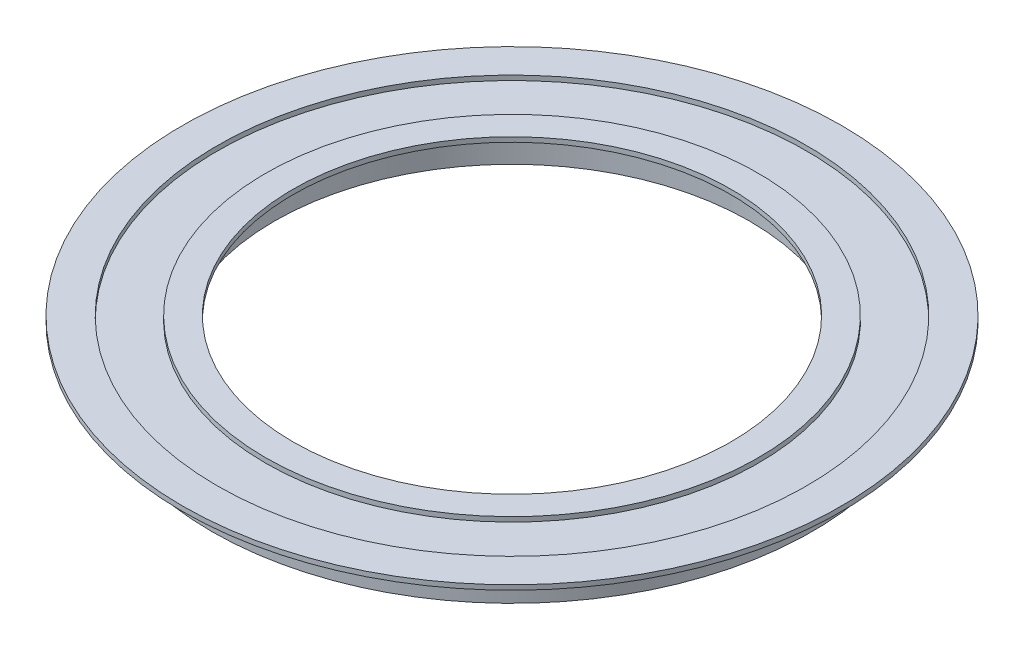
SolidWorks part; units mm, degrees
ref_plane "Front Plane" through (0, 0, 0) normal (0, 0, 1) x (1, 0, 0)
ref_plane "Top Plane" through (0, 0, 0) normal (0, 1, 0) x (1, 0, 0)
ref_plane "Right Plane" through (0, 0, 0) normal (1, 0, 0) x (0, 0, -1)
sketch "Sketch1" plane through (0, 0, 0) normal (0, 0, 1) x (1, 0, 0)
  line L0 (0, 0) -> (0, -15.1149) construction
  line L1 (63.1935, 160.5319) -> (69.3634, 160.5319)
  line L2 (63.1935, 160.5319) -> (-63.1935, 160.5319) construction
  line L3 (102, 160.5319) -> (-102, 160.5319) construction
  line L4 (69.3634, 160.5319) -> (69.3634, 161.5319)
  line L5 (69.3634, 161.5319) -> (62.0337, 161.5319)
  line L6 (63.1935, 160.5319) -> (63.1935, 153.779)
  line L7 (63.1935, 153.779) -> (-63.1935, 153.779) construction
  line L8 (63.1935, 153.779) -> (50, 153.779)
  line L10 (50, 153.779) -> (50, 160.5319)
  line L13 (50, 160.5319) -> (-50, 160.5319) construction
  line L14 (50, 160.5319) -> (62.0337, 160.5319)
  line L15 (62.0337, 160.5319) -> (62.0337, 161.5319)
  line L17 (46.0812, 160.568) -> (51.8531, 160.568)
  line L18 (46.0812, 160.568) -> (46.0812, 161.568)
  line L19 (46.0812, 161.568) -> (51.8531, 161.568)
  line L20 (51.8531, 160.568) -> (51.8531, 161.568)
revolve "Revolve1" add sketch "Sketch1" angle 360 about L0
